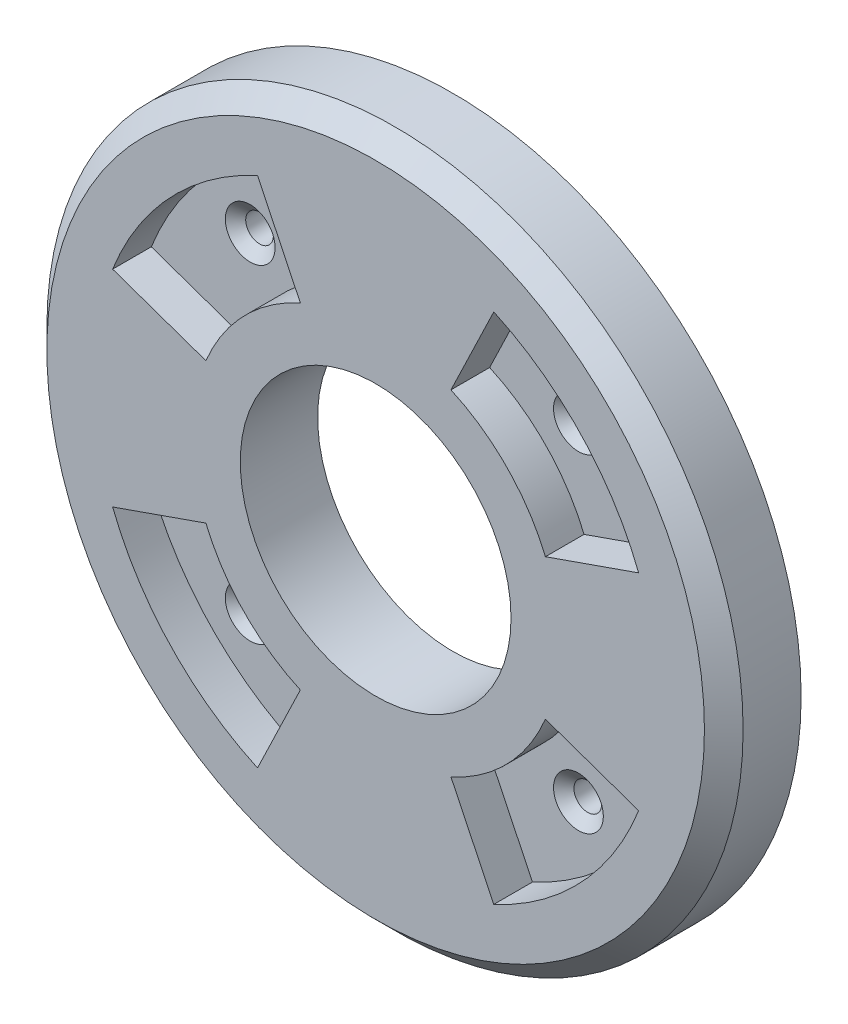
from build123d import *

# Parameters (mm, degrees)
SKETCH1_R                                           = 90
SKETCH1_R_2                                         = 35
BOSS_EXTRUDE1_DEPTH                                 = 20
CUT_EXTRUDE1_DEPTH                                  = 10
CHAMFER1_SIZE                                       = 5
CSK_FOR_1_4_FLAT_HEAD_MACHINE_SCREW_100_D           = 7.14248
CSK_FOR_1_4_FLAT_HEAD_MACHINE_SCREW_100_CSINK_D     = 12.8778
CSK_FOR_1_4_FLAT_HEAD_MACHINE_SCREW_100_CSINK_ANGLE = 100
MIRROR2_COPY_1_D                                    = 7.14248
MIRROR2_COPY_1_CSINK_D                              = 12.8778
MIRROR2_COPY_1_CSINK_ANGLE                          = 100


with BuildPart() as part:
    # Sketch1 → Boss-Extrude1 (new body)
    with BuildSketch(Plane.XY):
        Circle(SKETCH1_R)
        Circle(SKETCH1_R_2, mode=Mode.SUBTRACT)
    extrude(amount=BOSS_EXTRUDE1_DEPTH)

    # Sketch2 → Cut-Extrude1 (cut)
    with BuildSketch(Plane.XY.offset(20)):
        with BuildLine():
            Line((-19.468288874, 43.327078465), (-30.54243357, 66.327225141))
            ThreePointArc((-30.54243357, 66.327225141), (-53.118804443, 50.105225854), (-67.996083401, 26.620925706))
            Line((-67.996083401, 26.620925706), (-43.882710923, 18.181245339))
            ThreePointArc((-43.882710923, 18.181245339), (-34.079547015, 33.088283051), (-19.468288874, 43.327078465))
        make_face()
        with BuildLine():
            Line((43.882710923, 18.181245339), (67.996083401, 26.620925706))
            ThreePointArc((67.996083401, 26.620925706), (53.118804443, 50.105225854), (30.54243357, 66.327225141))
            Line((30.54243357, 66.327225141), (19.468288874, 43.327078465))
            ThreePointArc((19.468288874, 43.327078465), (34.079547015, 33.088283051), (43.882710923, 18.181245339))
        make_face()
        with BuildLine():
            Line((19.468288874, -43.327078465), (30.54243357, -66.327225141))
            ThreePointArc((30.54243357, -66.327225141), (53.118804443, -50.105225854), (67.996083401, -26.620925706))
            Line((67.996083401, -26.620925706), (43.882710923, -18.181245339))
            ThreePointArc((43.882710923, -18.181245339), (34.079547015, -33.088283051), (19.468288874, -43.327078465))
        make_face()
        with BuildLine():
            Line((-43.882710923, -18.181245339), (-67.996083401, -26.620925706))
            ThreePointArc((-67.996083401, -26.620925706), (-53.118804443, -50.105225854), (-30.54243357, -66.327225141))
            Line((-30.54243357, -66.327225141), (-19.468288874, -43.327078465))
            ThreePointArc((-19.468288874, -43.327078465), (-34.079547015, -33.088283051), (-43.882710923, -18.181245339))
        make_face()
    extrude(amount=-CUT_EXTRUDE1_DEPTH, mode=Mode.SUBTRACT)

    # Chamfer1
    chamfer1_edges = [part.edges().sort_by_distance(p)[0] for p in [
        (-90, 0, 20),
    ]]
    chamfer(chamfer1_edges, length=CHAMFER1_SIZE)

    # CSK for 1/4 Flat Head Machine Screw (100)1 (through all)
    with Locations(Plane.XY.offset(10)):
        with Locations((-42.426406871, 42.426406871)):
            csk_for_1_4_flat_head_machine_screw_100 = CounterSinkHole(CSK_FOR_1_4_FLAT_HEAD_MACHINE_SCREW_100_D / 2, CSK_FOR_1_4_FLAT_HEAD_MACHINE_SCREW_100_CSINK_D / 2, counter_sink_angle=CSK_FOR_1_4_FLAT_HEAD_MACHINE_SCREW_100_CSINK_ANGLE)

    # Mirror1: CSK for 1/4 Flat Head Machine Screw (100)1 across plane
    add(csk_for_1_4_flat_head_machine_screw_100.mirror(Plane(origin=(0, 0, 0), x_dir=(0, 0, 1), z_dir=(1, 0, 0))), mode=Mode.SUBTRACT)

    # Mirror2: CSK for 1/4 Flat Head Machine Screw (100)1 across plane
    add(csk_for_1_4_flat_head_machine_screw_100.mirror(Plane.ZX), mode=Mode.SUBTRACT)

    # Mirror2 copy 1 (through all)
    with Locations(Plane(origin=(0, 0, 10), x_dir=(-1, 0, 0), z_dir=(0, 0, 1))):
        with Locations((-42.426406871, 42.426406871)):
            CounterSinkHole(MIRROR2_COPY_1_D / 2, MIRROR2_COPY_1_CSINK_D / 2, counter_sink_angle=MIRROR2_COPY_1_CSINK_ANGLE)


solid = part.part
